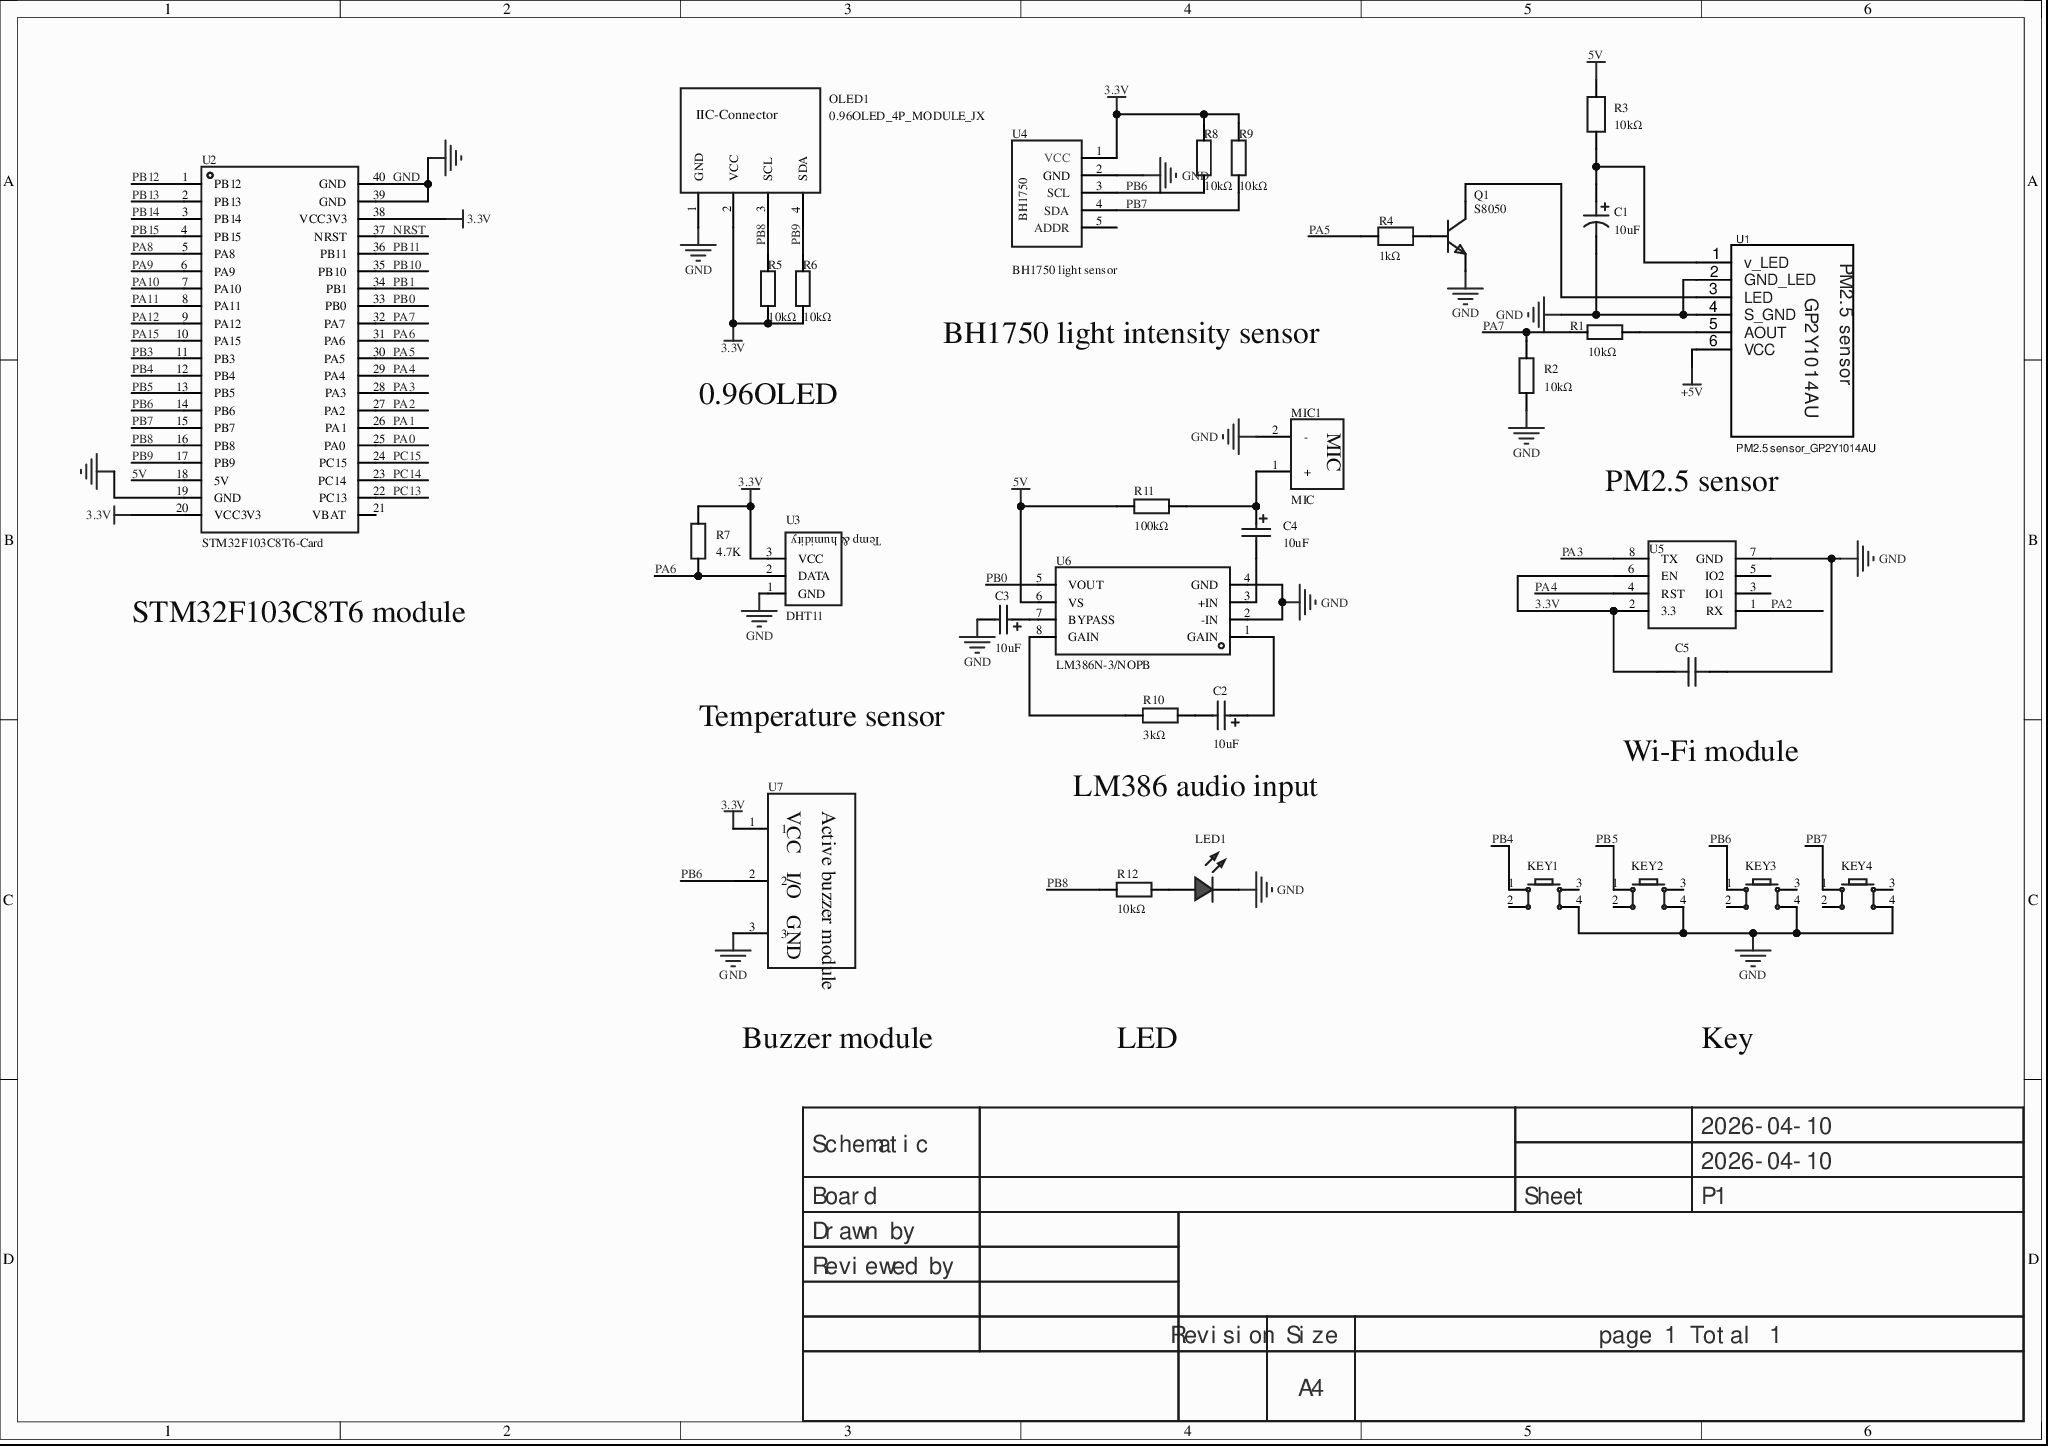
[diagram p0: MISC52092-3.schdoc]
# Altium project MISC52092-2.PrjPcb
1 sheet, 32 parts. Net scope: global (net labels, ports and power ports of the same name join across sheets).
Board file: MISC52092.pcbdoc

## Sheet MISC52092-3.schdoc
size 297 x 209 mm; Version: V1.0; @Project Name: MISC52092; @Update Date: 2026-04-10; @Create Date: 2026-04-10; @Board Name: MISC52092; @Create Time: 15:27:49; @Page Count: 1; @Page No: 1; @Schematic Name: MISC52092; @Update Time: 15:27:49; Size: A4

### Parts
C1  10uF  [CAP-TH_BD5.0-P2.00-D0.5-FD]
C2  10uF  [C_Ele_SMD_3x5.4mm]
C3  10uF  [C_Ele_SMD_3x5.4mm]
C4  10uF  [C_Ele_SMD_3x5.4mm]
C5  5pF  [CAP-TH_L5.0-W3.0-P5.00-D0.6]  (value not drawn)
KEY1  (no value)  [SW-TH_4P-L6.0-W6.0-P4.50-LS6.5]
KEY2  (no value)  [SW-TH_4P-L6.0-W6.0-P4.50-LS6.5]
KEY3  (no value)  [SW-TH_4P-L6.0-W6.0-P4.50-LS6.5]
KEY4  (no value)  [SW-TH_4P-L6.0-W6.0-P4.50-LS6.5]
LED1  (no value)  [LED_TH-3mm]
MIC1  MIC  [MIC-TH_BD6.0-P2.00]
OLED1  0.96OLED_4P_MODULE_JX  [0.96OLED_4P]
Q1  S8050  [TO-92-3_L4.5-W3.5-P1.27-L]
R1  10kΩ  [Res_1/4W]
R2  10kΩ  [Res_1/4W]
R3  10kΩ  [RES-TH_BD2.7-L6.2-P10.20-D0.4]
R4  1kΩ  [RES-TH_BD2.7-L6.2-P10.20-D0.4]
R5  10kΩ  [Res_1/4W]
R6  10kΩ  [Res_1/4W]
R7  4.7K  [Res_1/4W]
R8  10kΩ  [Res_1/4W]
R9  10kΩ  [Res_1/4W]
R10  3kΩ  [Res_1/4W]
R11  100kΩ  [Res_1/4W]
R12  10kΩ  [Res_1/4W]
U1  PM2.5 sensor_GP2Y1014AU  [PM2.5传感器_GP2Y1014AU]
U2  STM32F103C8T6-Card  [CONN-TH_L53.3-W22.9_STM32F103C8T6-CARD]
U3  DHT11  [DHT11]
U4  Device: BH1750 light sensor  [BH1750光照传感器]
U5  (no value)  [ESP8266-1]
U6  LM386N-3/NOPB  [DIP-8_L9.8-W6.6-P2.54-LS7.6-BL]
U7  (no value)  [有源蜂鸣器模块]

### Nets
3.3V: C5.1 OLED1.2(VCC) R5.1 R6.1 R7.2 R8.2 R9.2 U2.20(VCC3V3) U2.38(VCC3V3) U3.3(VCC) U4.1(VCC) U5.2(3.3) U5.6(EN) U7.1
5V: R3.2 R11.1 U2.18(5V) U6.6(VS)
+5V: U1.6(VCC)
GND: C1.2 C3.2 C5.2 KEY1.4 KEY2.4 KEY3.4 KEY4.4 LED1.2(A) MIC1.2(-) OLED1.1(GND) Q1.1(E) R2.1 U1.2(GND_LED) U1.4(S_GND) U2.19(GND) U2.39(GND) U2.40(GND) U3.1(GND) U4.2(GND) U5.7(GND) U6.2(-IN) U6.4(GND) U7.3
NRST: U2.37(NRST)
PA0: U2.25(PA0)
PA1: U2.26(PA1)
PA2: U2.27(PA2) U5.1(RX)
PA3: U2.28(PA3) U5.8(TX)
PA4: U2.29(PA4) U5.4(RST)
PA5: R4.1 U2.30(PA5)
PA6: R7.1 U2.31(PA6) U3.2(DATA)
PA7: R1.1 R2.2 U2.32(PA7)
PA8: U2.5(PA8)
PA9: U2.6(PA9)
PA10: U2.7(PA10)
PA11: U2.8(PA11)
PA12: U2.9(PA12)
PA15: U2.10(PA15)
PB0: U2.33(PB0) U6.5(VOUT)
PB1: U2.34(PB1)
PB3: U2.11(PB3)
PB4: KEY1.1 U2.12(PB4)
PB5: KEY2.1 U2.13(PB5)
PB6: KEY3.1 R8.1 U2.14(PB6) U4.3(SCL) U7.2
PB7: KEY4.1 R9.1 U2.15(PB7) U4.4(SDA)
PB8: OLED1.3(SCL) R5.2 R12.2 U2.16(PB8)
PB9: OLED1.4(SDA) R6.2 U2.17(PB9)
PB10: U2.35(PB10)
PB11: U2.36(PB11)
PB12: U2.1(PB12)
PB13: U2.2(PB13)
PB14: U2.3(PB14)
PB15: U2.4(PB15)
PC13: U2.22(PC13)
PC14: U2.23(PC14)
PC15: U2.24(PC15)
NetC1_1: C1.1 R3.1 U1.1(v_LED)
NetC2_1: C2.1 U6.1(GAIN)
NetC2_2: C2.2 R10.2
NetC3_1: C3.1 U6.7(BYPASS)
NetC4_1: C4.1 MIC1.1(+) R11.2
NetC4_2: C4.2 U6.3(+IN)
NetLED1_1: LED1.1(C) R12.1
NetQ1_2: Q1.2(B) R4.2
NetQ1_3: Q1.3(C) U1.3(LED)
NetR1_2: R1.2 U1.5(AOUT)
NetR10_1: R10.1 U6.8(GAIN)

Not connected (* = marked no-connect by the designer): KEY1 2* 3*; KEY2 2* 3*; KEY3 2* 3*; KEY4 2* 3*; U2 21(VBAT); U4 5(ADDR); U5 3(IO1) 5(IO2)

### Notes on the sheet
- BH1750 light intensity sensor
- 0.96OLED
- (near U5) PM2.5 sensor
- STM32F103C8T6 module
- Temperature sensor
- (near C5) Wi-Fi module
- LM386 audio input
- Buzzer module
- LED
- Key
- 2026-04-10
- Schematic
- Board
- Sheet
- P1
- Drawn by
- Reviewed by
- Revision
- Size
- A4
- page 1 Total 1

### Library data of the parts
C1 = SHG63V10UF03EC0822: Capacitance:10uF;Tolerance:±20%;Rated voltage:63V;; 3D Model: aba3b94bdab6406eb4f45c9c765c730e0819f05c4eef4c71ace90d822a990e87; 3D Model Transform: 196.85,196.517,0,0,0,0,0,0,-196.85; Tolerance: ±20%; Voltage Rating: 63V; AddInBom: yes; Symbol: SHG63V10UF03EC0822; Device: SHG63V10UF03EC0822; LCSC Part Name: 停产 10uF ±20% 63V; Supplier Part: C5263880; Manufacturer Part: SHG63V10UF03EC0822; Supplier Footprint: 插件,D5xL11mm; JLCPCB Part Class: Extended Part; Datasheet: https://atta.szlcsc.com/upload/public/pdf/source/20221206/74D9A2C5191757C58A566DD8357A6A8B.pdf; Supplier: LCSC; Value: 10uF; Diameter: 5mm; Height - Seated (Max): 11mm; ConvertToPcb: yes; FootprintName: CAP-TH_BD5.0-P2.00-D0.5-FD; ModelName: CAP-TH_BD5.0-P2.00-D0.5-FD
C2-C4 = C_Ele_SMD_3x5.4mm: Symbol: CAP; AddInBom: yes; ModelId: 0132c3d3fdbf4fd987f710a97e7a5b5d0819f05c4eef4c71ace90d822a990e87; ModelName: CAP-SMD_BD3.0-L3.3-W3.3-H5.3; ModelTransform: 129.9,149.58,209.06,-90,0,0,0,0,0; Device: C_Ele_SMD_3x5.4mm; Supplier Footprint: SMD,3x5.4mm; ConvertToPcb: yes; FootprintName: C_Ele_SMD_3x5.4mm; Value: 10uF
C5 = DCC509D20COHF6FJ5A0: Capacitance:5pF;Rated voltage:50V;Temp coefficient:COH;; Manufacturer: SHM(南方宏明); 3D Model: 333cb9c3486d40e5b0f1e9901eb76dd90819f05c4eef4c71ace90d822a990e87; 3D Model Transform: 236.00874,118.5037,0,0,0,0,0,0,-196.85; Voltage Rating: 50V; Pin Spacing: 5mm; Temperature Coefficient: COH; AddInBom: yes; Symbol: DCC509D20COHF6FJ5A0; Device: DCC509D20COHF6FJ5A0; LCSC Part Name: ±0.5PF 5pF 50V; Supplier Part: C2896136; Manufacturer Part: DCC509D20COHF6FJ5A0; Supplier Footprint: 插件,P=5mm; JLCPCB Part Class: Extended Part; Datasheet: https://item.szlcsc.com/datasheet/DCC509D20COHF6FJ5A0/3138685.html; Supplier: LCSC; Value: 5pF; Diameter: 5mm; ConvertToPcb: yes; FootprintName: CAP-TH_L5.0-W3.0-P5.00-D0.6; ModelName: CAP-TH_L5.0-W3.0-P5.00-D0.6
KEY1-KEY4 = Key_TH_6x6x6: Contact current:50mA;Rated voltage(DC):12V;Insulation resistance:100MΩ;Circuit structure:single pole single throw;Mounting:through-hole;Button shape:round;Button/cap colour:black;Actuation force:260gf@±30gf;Operating temperature:-25℃~+70℃;Pin style:PC pin;Switch length:6mm;Switch width:6mm;Switch height:6mm;With bracket:no;; Symbol: Tactile switch; 3D Model: 20eee248bc684ccd8cbdbb1d0d91ec6f0819f05c4eef4c71ace90d822a990e87; 3D Model Transform: 236.22,323.03,0,90,0,0,0,0,-137.795; AddInBom: yes; ModelName: SW-TH_4P-L6.0-W6.0-H5.0-LS6.5-P4.50; Device: Key_TH_6x6x6; Supplier Footprint: 插件; ConvertToPcb: yes; FootprintName: SW-TH_4P-L6.0-W6.0-P4.50-LS6.5
LED1 = LED_TH-R_3mm: 3D Model: a497c992633541038a38947cdc58012f0819f05c4eef4c71ace90d822a990e87; 3D Model Transform: 141.274,153.327,0,0,0,0,-5.984,0,-137.795; ConvertToPcb: yes; ModelName: LED-TH-3mm_R; Symbol: LED_TH-R; Device: LED_TH-R_3mm; Supplier Footprint: 插件; AddInBom: yes; FootprintName: LED_TH-3mm
MIC1 = MIC: Symbol: MIC_C9900023869; AddInBom: yes; ModelId: 3d52db69e70846c48297d609207968340819f05c4eef4c71ace90d822a990e87; ModelTransform: 228.346,228.21852,0,0,0,0,0,0,-78.74; Device: MIC; LCSC Part Name: MIC; SupplierPart: C9900023869; ManufacturerPart: MIC; Supplier Footprint: THrough hole; JLCPCB Part Class: Extended Part; Supplier: LCSC; ConvertToPcb: yes; FootprintName: MIC-TH_BD6.0-P2.00; ModelName: MIC-TH_BD6.0-P2.00
OLED1 = 0.96OLED_4P_MODULE_JX: 3D Model: 79c000fdb68d45a296c2e9bedf4f90550819f05c4eef4c71ace90d822a990e87; 3D Model Transform: 1393.69792,1318.895,0,0,0,0,0,-560.079,-137.795; AddInBom: yes; Symbol: 0.96OLED_4P_MODULE_JX; Device: 0.96OLED_4P_MODULE_JX; LCSC Part Name: 0.96OLED_4P_MODULE_JX; Supplier Part: C9900004566; Manufacturer Part: 0.96OLED_4P_MODULE_JX; Supplier Footprint: 插件; JLCPCB Part Class: Extended Part; Supplier: LCSC; ConvertToPcb: yes; FootprintName: 0.96OLED_4P; ModelName: 0.96OLED_4P
Q1 = S8050_C2931492: Transistor type:NPN;Collector current(Ic):500mA;Collector-emitter breakdown voltage(Vceo):25V;Power dissipation(Pd):625mW;DC current gain(hFE):160@50mA,1V;; Manufacturer: JSMSEMI(杰盛微); 3D Model: 45fa6cddef3743c6aacf8db740a3bc4c0819f05c4eef4c71ace90d822a990e87; 3D Model Transform: 177.165,137.795,0,0,0,0,0,29.528,-98.425; type: NPN; Current - Collector(Ic): 500mA; Collector - Emitter Voltage VCEO: 25V; Pd - Power Dissipation: 625mW; Transition frequency(fT): 150MHz; Current - Collector Cutoff: 100nA; Vce Saturation(VCE(sat)): 600mV@500mA,50mA; Emitter-Base Voltage(Vebo): 5V; AddInBom: yes; Symbol: S8050_C2931492; Device: S8050_C2931492; LCSC Part Name: NPN 电流:500mA 电压:25V; Supplier Part: C2931492; Manufacturer Part: S8050; Supplier Footprint: TO-92; JLCPCB Part Class: Extended Part; Datasheet: https://item.szlcsc.com/datasheet/S8050/3272796.html; Supplier: LCSC; DC Current Gain: 160@50mA,1V; ConvertToPcb: yes; FootprintName: TO-92-3_L4.5-W3.5-P1.27-L; ModelName: TO-92-3_L4.5-W3.5-P1.27-L
R1 R2 R5-R12 = Res_AXIAL-1/4W: Symbol: Resistor; 3D Model: 463263665006444ab7a47bd11b0cf9560819f05c4eef4c71ace90d822a990e87; 3D Model Transform: 427.165,94.32816,0,0,0,0,0,0,-196.85; AddInBom: yes; ModelName: RES-TH_BD2.4-L6.3-P10.30-D0.6; Device: Res_AXIAL-1/4W; Supplier Footprint: 轴向引线; ConvertToPcb: yes; FootprintName: Res_1/4W
  R1 R2 R5 R6 R8 R9 R12: Value: 10kΩ
  R7: Value: 4.7K
  R10: Value: 3kΩ
  R11: Value: 100kΩ
R3 = MF1/4W-10K±1%-ST52: Resistor type:metal film resistor;Resistance:10kΩ;Tolerance:±1%;Power:250mW;Temp coefficient:±100ppm/℃;; Manufacturer: VO(翔胜); 3D Model: f91fbe0e2e6f409498f09f811e4616fe0819f05c4eef4c71ace90d822a990e87; 3D Model Transform: 417.322,106.221,0,0,0,0,0,0,-196.85; Tolerance: ±1%; Voltage-Supply(Max): 250V; Power(Watts): 250mW; AddInBom: yes; Symbol: MF1/4W-10K±1%-ST52; Device: MF1/4W-10K±1%-ST52; LCSC Part Name: 金属膜电阻 10kΩ ±1% 250mW; Supplier Part: C2903232; Manufacturer Part: MF1/4W-10K±1%-ST52; Supplier Footprint: 插件,D2.7xL6.2mm; JLCPCB Part Class: Extended Part; Datasheet: https://item.szlcsc.com/datasheet/MF1%252F4W-10K%25C2%25B11%2525-ST52/3158983.html; Supplier: LCSC; Type: Metal film resistor; Value: 10kΩ; Temperature Coefficient: ±100ppm/℃; Operating Temperature: -55℃~+155℃; ConvertToPcb: yes; FootprintName: RES-TH_BD2.7-L6.2-P10.20-D0.4; ModelName: RES-TH_BD2.7-L6.2-P10.20-D0.4
R4 = MF1/4W-1K±1%-ST52: Resistor type:metal film resistor;Resistance:1kΩ;Tolerance:±1%;Power:250mW;Temp coefficient:±100ppm/℃;; Manufacturer: VO(翔胜); 3D Model: f91fbe0e2e6f409498f09f811e4616fe0819f05c4eef4c71ace90d822a990e87; 3D Model Transform: 417.322,106.221,0,0,0,0,0,0,-196.85; Tolerance: ±1%; Voltage-Supply(Max): 250V; Power(Watts): 250mW; AddInBom: yes; Symbol: MF1/4W-1K±1%-ST52; Device: MF1/4W-1K±1%-ST52; LCSC Part Name: 金属膜电阻 1kΩ ±1% 250mW; Supplier Part: C2903245; Manufacturer Part: MF1/4W-1K±1%-ST52; Supplier Footprint: 插件,D2.7xL6.2mm; JLCPCB Part Class: Extended Part; Datasheet: https://item.szlcsc.com/datasheet/MF1%252F4W-1K%25C2%25B11%2525-ST52/3158996.html; Supplier: LCSC; Type: Metal film resistor; Value: 1kΩ; Temperature Coefficient: ±100ppm/℃; Operating Temperature: -55℃~+155℃; ConvertToPcb: yes; FootprintName: RES-TH_BD2.7-L6.2-P10.20-D0.4; ModelName: RES-TH_BD2.7-L6.2-P10.20-D0.4
U1 = PM2.5传感器_GP2Y1014AU: Symbol: PM2.5 sensor_GP2Y1014AU; Device: PM2.5 sensor_GP2Y1014AU; FootprintName: PM2.5 sensor_GP2Y1014AU
U2 = STM32F103C8T6-Card: AddInBom: yes; Symbol: STM32F103C8T6-CARD; Device: STM32F103C8T6-Card; LCSC Part Name: STM32F103C8T6-Card; Supplier Part: C9900077949; Manufacturer Part: STM32F103C8T6-Card; Supplier Footprint: 插件; Supplier: LCSC; ConvertToPcb: yes; FootprintName: CONN-TH_L53.3-W22.9_STM32F103C8T6-CARD
U3 = DHT11: ConvertToPcb: yes; Symbol: DHT11; Device: DHT11; AddInBom: yes; FootprintName: DHT11
U4 = BH1750光照传感器: AddInBom: yes; Symbol: BH1750 light sensor; ConvertToPcb: yes; FootprintName: BH1750 light sensor
U5 = esp8266: esp8266 module pinout diagram; AddInBom: yes; Symbol: esp8266; Device: esp8266; ConvertToPcb: yes; FootprintName: ESP8266-1
U6 = LM386N-3/NOPB: Amplifier type:class AB;Speaker channels:mono;Output power:700mWx1@8Ω;Quiescent current(Iq):4mA;; Manufacturer: TI(德州仪器); AddInBom: yes; ModelId: db2af726fcec488f8bf8e467aca974b30819f05c4eef4c71ace90d822a990e87; ModelName: DIP-8_L9.8-W6.6-H3.5-LS7.62-P2.54; ModelTransform: 385.826,311.8104,0,0,0,0,-1.693,0,-137.795; Class: Class AB amplifier; Speaker Channels: Mono; Voltage - Supply: 4V~12V; Total Harmonic Distortion + Noise (THD+N): 0.2%; Quiescent Current: 4mA; Power Supply Rejection Ratio (PSRR): 50dB; Symbol: LM386N-3; Device: LM386N-3/NOPB; LCSC Part Name: 700mW单声道AB类音频功率放大器; SupplierPart: C139428; ManufacturerPart: LM386N-3/NOPB; Supplier Footprint: PDIP-8; JLCPCB Part Class: Extended Part; Supplier: LCSC; ConvertToPcb: yes; FootprintName: DIP-8_L9.8-W6.6-P2.54-LS7.6-BL; Output Power: 700mWx1@8Ω; Operating Temperature: 0℃~+70℃
U7 = 有源蜂鸣器模块: Symbol: Active buzzer module; AddInBom: yes; Device: Active buzzer module; ConvertToPcb: yes; FootprintName: Active buzzer module